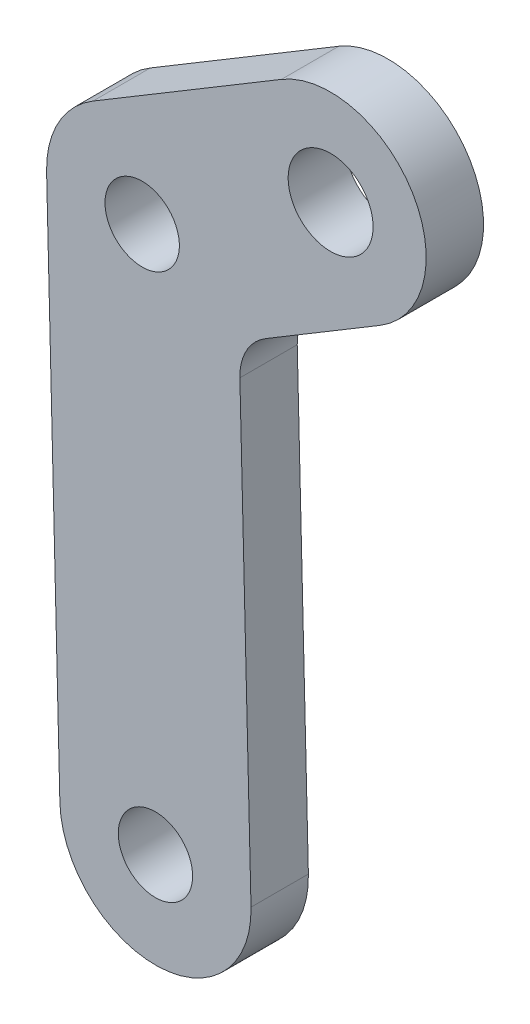
SolidWorks part; units mm, degrees
material "AISI 1045 钢，冷拔"
ref_plane "Front Plane" through (0, 0, 0) normal (0, 0, 1) x (1, 0, 0)
ref_plane "Top Plane" through (0, 0, 0) normal (0, 1, 0) x (1, 0, 0)
ref_plane "Right Plane" through (0, 0, 0) normal (1, 0, 0) x (0, 0, -1)
sketch "Sketch1" plane through (0, 0, 0) normal (0, 0, 1) x (1, 0, 0)
  line L0 (0, 37.7743) -> (0, 34.2743) construction
  line L1 (0, 37.7743) -> (-0.0861, 34.2754) construction
  line L2 (0, 37.7743) -> (0, -32.8501) construction
  line L3 (0, 37.7743) -> (1.9571, -41.7364) construction
  line L4 (1.25, -13.0102) -> (0, -13.0102) construction
  line L5 (-8.9973, 37.5528) -> (-7.7473, -13.2317)
  line L6 (1.25, -13.0102) -> (39.7517, -13.0102) construction
  line L7 (9.198, 29.8412) -> (10.2473, -12.7887)
  line L8 (14.2, 55.2356) -> (14.2, 34.9678) construction
  line L9 (11.8073, 29.9643) -> (14.2009, 29.9643) construction
  line L10 (22.3678, 40.6971) -> (11.6272, 34.2562)
  line L11 (19.2035, 29.9643) -> (20.5271, 29.9643) construction
  line L12 (14.2, 24.9608) -> (14.2, 10.9614) construction
  line L13 (-4.6286, 45.4928) -> (13.1122, 56.1315)
  circle A0 centre (0, 37.7743) radius 3.5
  circle A2 centre (1.25, -13.0102) radius 3.5
  arc A3 (-4.6286, 45.4928) -> (-8.9973, 37.5528) centre (0, 37.7743) ccw
  arc A4 (-7.7473, -13.2317) -> (10.2473, -12.7887) centre (1.25, -13.0102) ccw
  arc A5 (11.6272, 34.2562) -> (9.198, 29.8412) centre (14.2009, 29.9643) ccw
  arc A6 (0, 28.7743) -> (0.2215, 28.777) centre (0, 37.7743) ccw
  circle A7 centre (17.74, 48.4143) radius 4
  arc A8 (22.3678, 40.6971) -> (13.1122, 56.1315) centre (17.74, 48.4143) ccw
  dimension "D2" = 50.7845
  dimension "D3" = 7
  dimension "D4" = 7
  dimension "D5" = 18
  dimension "D6" = 18
  dimension "D10" = 30.95
  dimension "D12" = 17.74
  dimension "D13" = 10.64
  dimension "D1" = 1.41
  dimension "D7" = 271.41
  dimension "D8" = 14.2
  dimension "D9" = 7.81
  dimension "D11" = 30.95
extrude "Boss-Extrude1" add sketch "Sketch1" along normal blind 5.4
